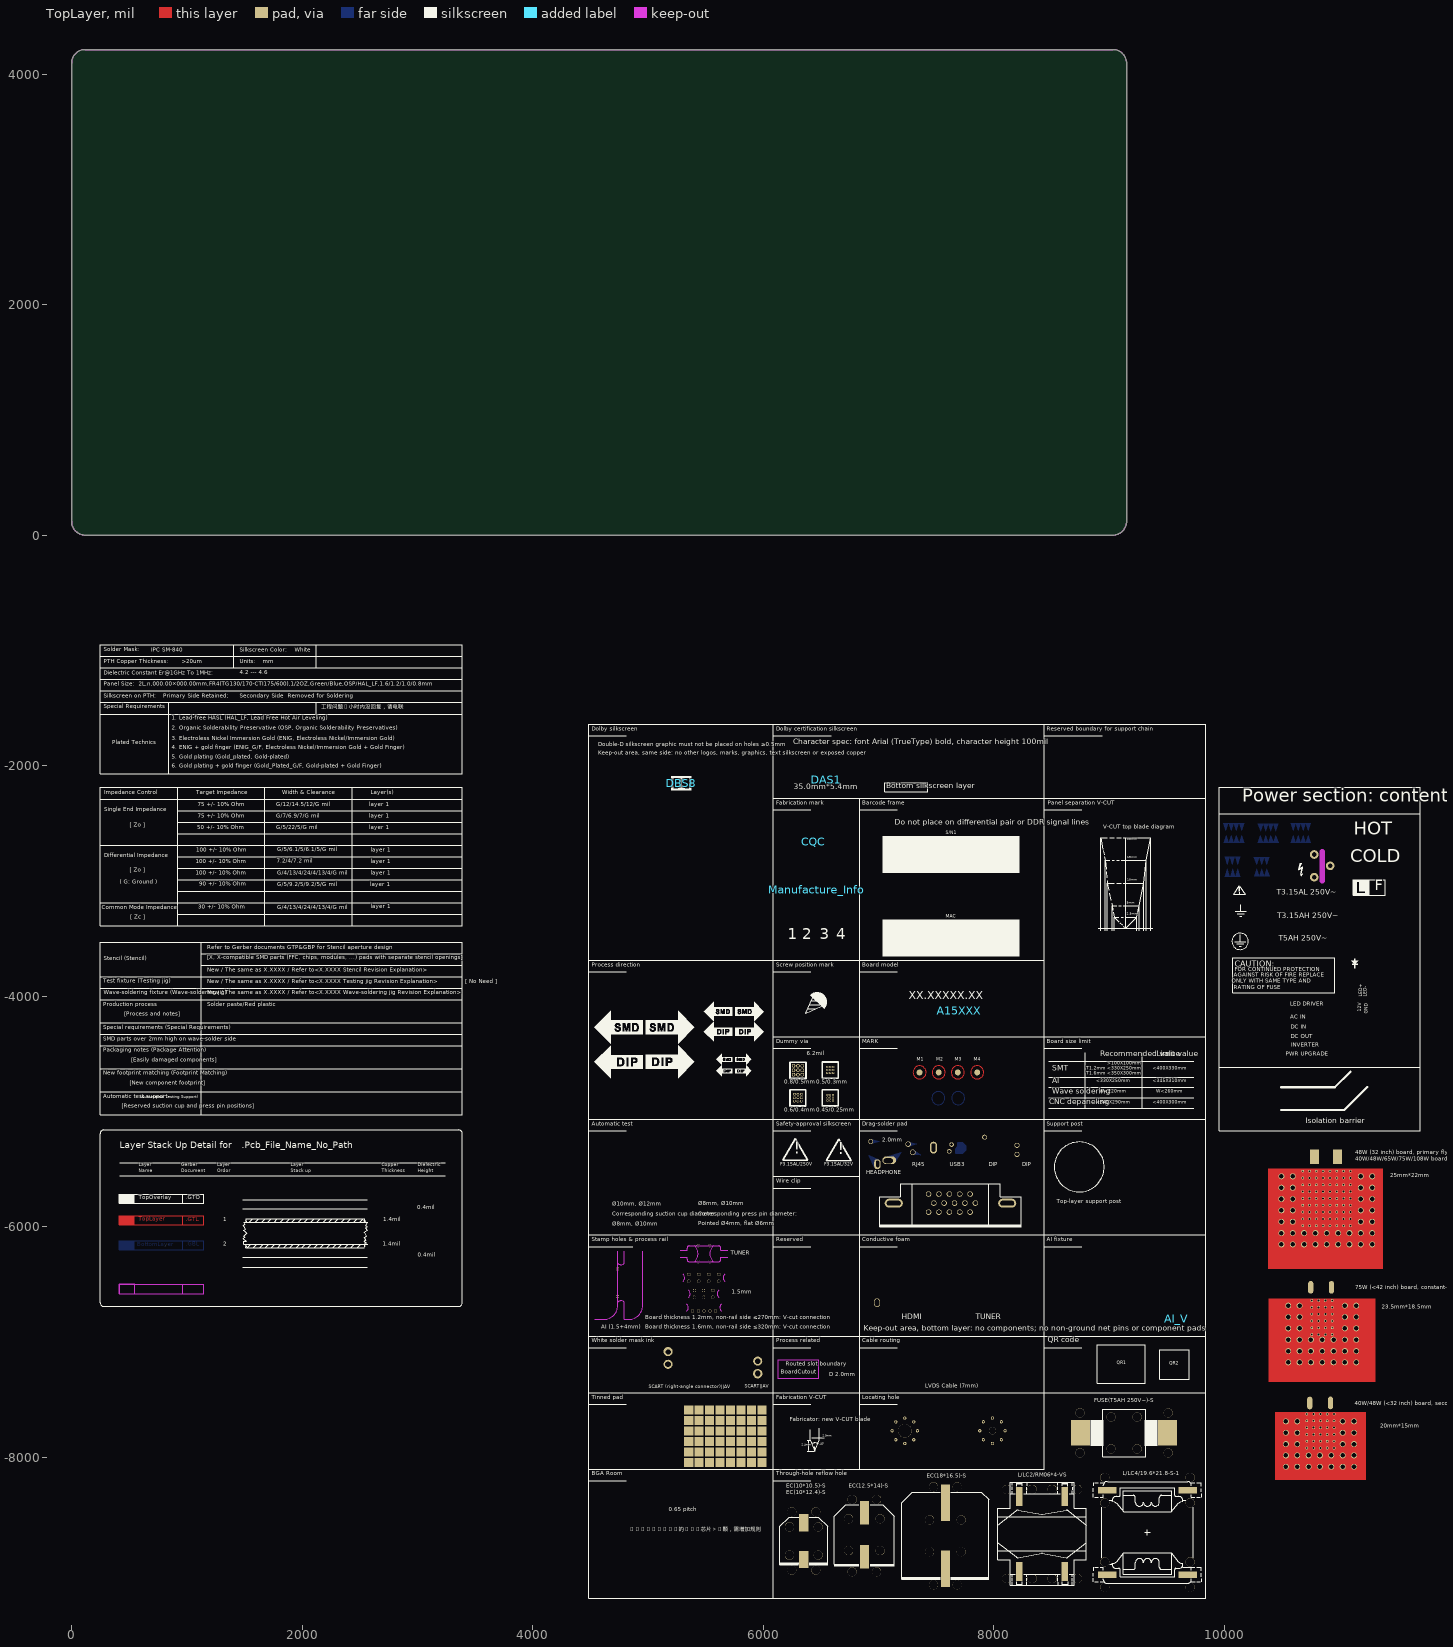
[diagram p0: TopLayer view]
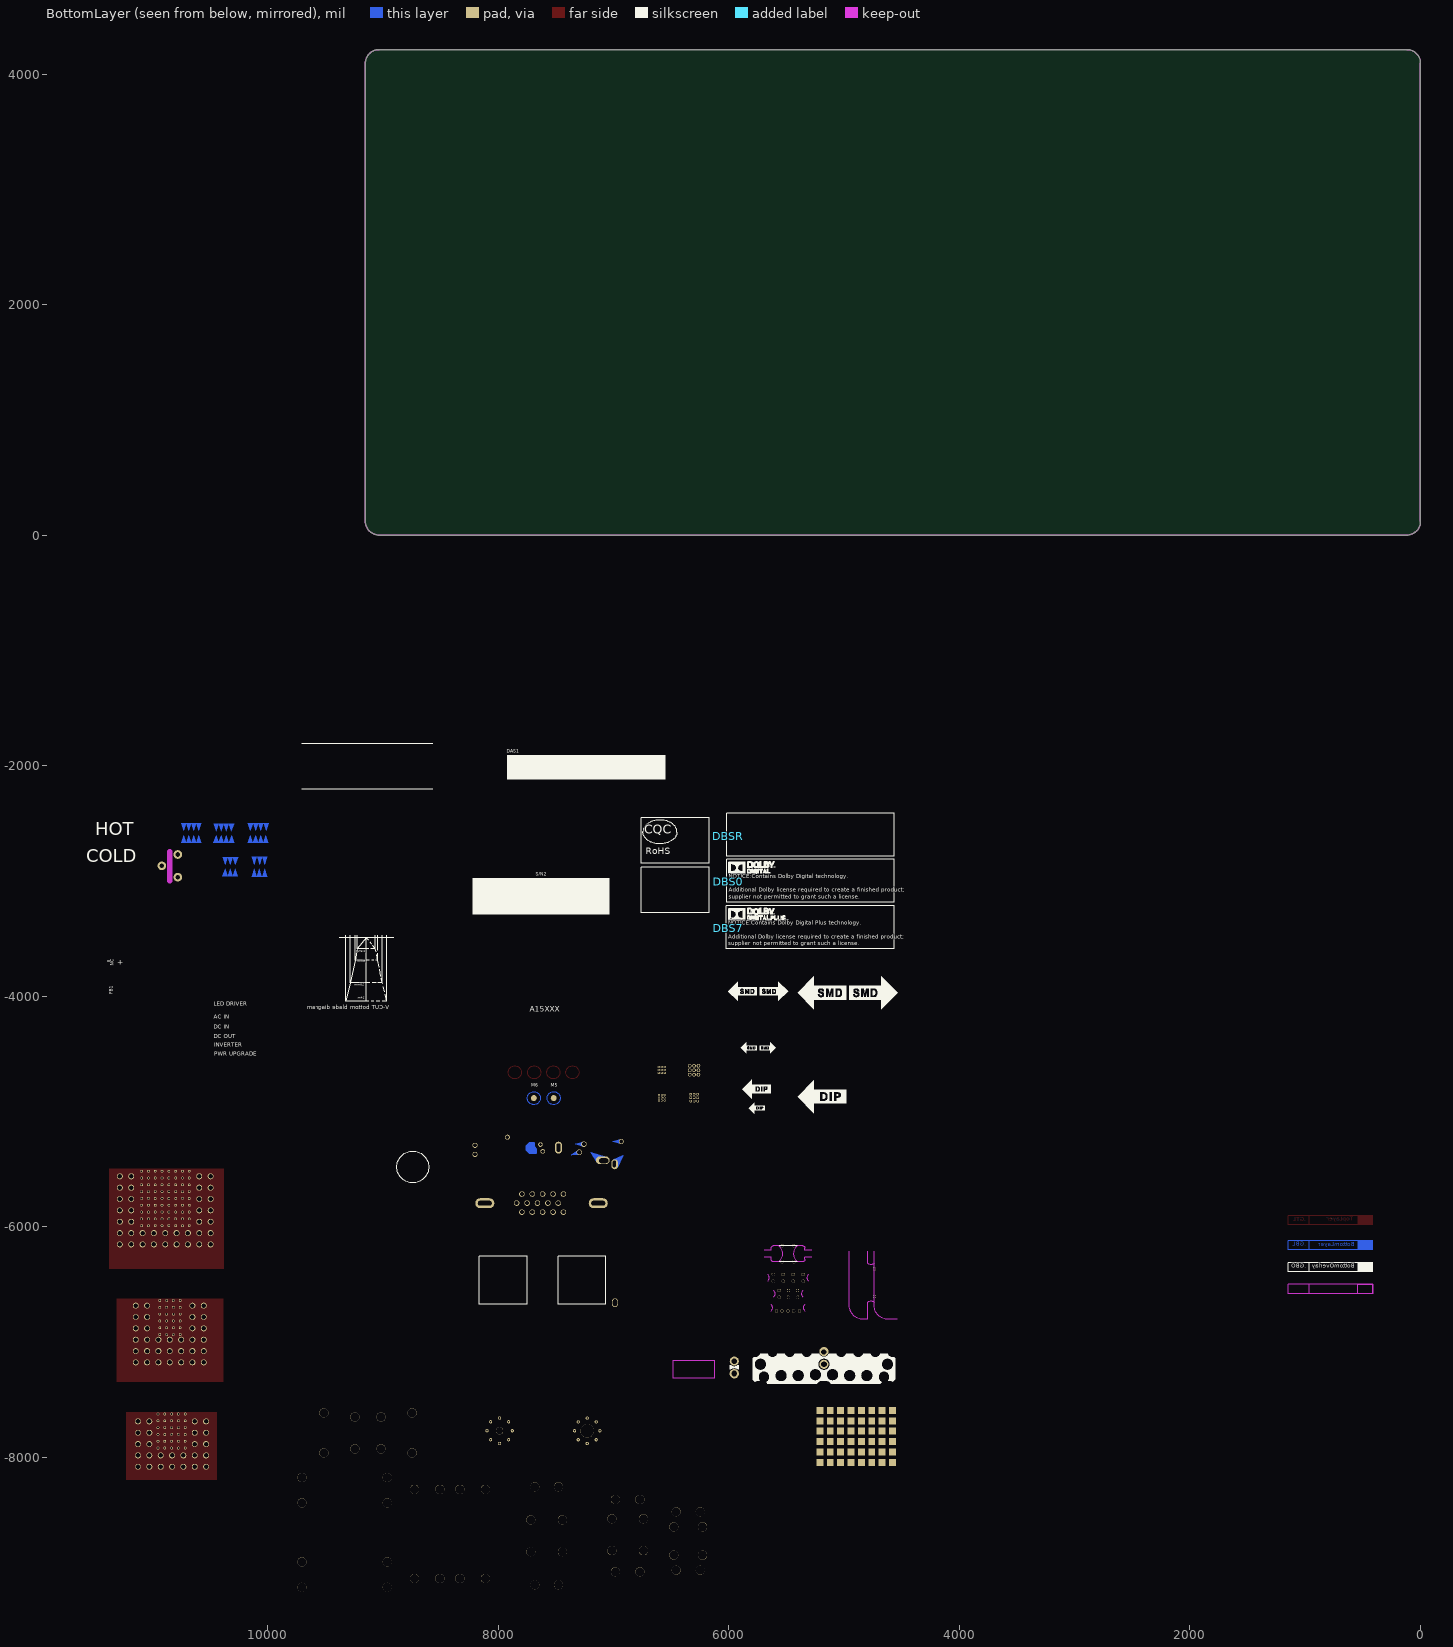
[diagram p1: BottomLayer view, seen from below]
# Altium PCB MISC86383.PcbDoc (part 1 of 2)
Units mil, origin at the board's own origin, x right, y up, seen from the top; angles counter-clockwise.
Board outline 9153.54 x 4212.6 mil, 2 copper layers (TopLayer, BottomLayer), stack 61.855 mil thick; 21 components, 2 nets, 540 pads, 0 vias.

## Layer stack, top to bottom
TopLayer: signal copper 1.4
Dielectric: core 59.055, FR-4, Dk 4.8
BottomLayer: signal copper 1.4

## Board outline
0,118.11 ccw(c118.11,118.11) 118.11,0 9035.43,0 9035.44,0 ccw(c9035.44,118.11) 9153.55,118.11 9153.55,4094.49 ccw(c9035.44,4094.49) 9035.44,4212.6 118.11,4212.6 ccw(c118.11,4094.49) 0,4094.49
cut-out: 6125.57,-7157.75 6125.57,-7314.38 6481.71,-7314.38 6481.71,-7157.75

## Design rules (kind name [scope] priority, off if disabled: settings)
Clearance ■KEEPOUT_18mil [(IsTrack Or IsArc) And (AsMM(Width) < 1) And IsKeepOut vs Not IsPad] p1: gap=18
Clearance ■HOT_7.2mm [InNetClass('HOT') vs InNetClass('All Nets') And (Not InNetClass('HOT'))] p2: gap=283.46
Clearance ■DFM_NPTH_10mil [(IsPadHoleValid And (PadIsPlated=false) Or IsPad And ((AsMM(PadXSize_AllLayers) < 1) or (AsMM(PadYSize_AllLayers) < 1 )) And IsKeepout) OR HasFootprintPad('ASSE*','0') vs Not IsPad] p3: gap=10
Clearance ■DFM_20mil [(IsTrack or IsArc or IsPad) And IsKeepOut vs IsTrack or IsArc or InPoly] p4: gap=20
Clearance ■C_RJ45_2mm [InNetClass('RJ45') vs Not InNetClass('RJ45') AND InNet('*')] p5: gap=78.74
Clearance ■VIA2VIA_6.2mil [(IsVia OR InPadClass('VIA5')) And Not ((IsVia OR InPadClass('VIA5')) And (AsMM(HoleDiameter) = 0.1)) vs (IsVia OR InPadClass('VIA5')) And Not ((IsVia OR InPadClass('VIA5')) And (AsMM(HoleDiameter) = 0.1))] p6: gap=6.2
Clearance ■V2V_BGA0p65_9p8mil [((IsVia OR InPadClass('VIA5')) And Not ((IsVia OR InPadClass('VIA5')) And (AsMM(HoleDiameter) = 0.1))) And (WithInRoom('BGA0p65-1') OR WithInRoom('BGA0p65-2')) vs ((IsVia OR InPadClass('VIA5')) And Not ((IsVia OR InPadClass('VIA5')) And (AsMM(HoleDiameter) = 0.1))) And (WithInRoom('BGA0p65-1') OR WithInRoom('BGA0p65-2'))] p7: gap=9.8
Clearance ■VIA2VIA_10.2mil [((IsVia OR InPadClass('VIA5')) And Not ((IsVia OR InPadClass('VIA5')) And (AsMM(HoleDiameter) = 0.1))) And Not (WithInRoom('BGA0p65-1') OR WithInRoom('BGA0p65-2')) vs ((IsVia OR InPadClass('VIA5')) And Not ((IsVia OR InPadClass('VIA5')) And (AsMM(HoleDiameter) = 0.1))) And Not (WithInRoom('BGA0p65-1') OR WithInRoom('BGA0p65-2'))] p8: gap=10.2
Clearance ■PWR_A12_8mil [((InNetClass('PWR_A12_8mil') or InNet('*12V*') or InNet('*24V*') or InNet('*PVCC*') or InNet('*19V*') or InNet('*AMP*POWER*') or InNet('*AMP*VCC*') or InNet('*LNB*')) And Not InNetClass('A12_8mil_EXC')) and Not IsPad vs Not InPoly] p9: gap=8
Clearance ■PS_L2All_3.2mm [InNet('L-1') vs InNet('*')] p10: gap=125.98
Clearance ■PS_L2LN_1.5mm [InNet('L') Or InNet('L-2') Or InNet('L-3') Or InNet('L-4') Or InNet('L-5') Or InNet('L-6') vs InNet('L-N') And Not(InNet('L') Or InNet('L-2') Or InNet('L-3') Or InNet('L-4') Or InNet('L-5') Or InNet('L-6'))] p11: gap=59.06
Clearance ■PS_N2LN_1.5mm [InNet('N') OR InNet('N-1') OR InNet('N-2') OR InNet('N-3') OR InNet('N-4') OR InNet('N-5') OR InNet('N-6') vs InNet('L-N') And Not (InNet('N') OR InNet('N-1') OR InNet('N-2') OR InNet('N-3') OR InNet('N-4') OR InNet('N-5') OR InNet('N-6'))] p12: gap=59.06
Clearance ■PS_L2LN_3mm [InNet('L') Or InNet('L-2') Or InNet('L-3') Or InNet('L-4') Or InNet('L-5') Or InNet('L-6') vs InNet('*') And Not (InNet('L-N') Or InNet('L') Or InNet('L-2') Or InNet('L-3') Or InNet('L-4') Or InNet('L-5') Or InNet('L-6') Or OnLayer('KeepOutLayer'))] p13: gap=118.11
Clearance ■PS_N2LN_3mm [InNet('N') OR InNet('N-1') OR InNet('N-2') OR InNet('N-3') OR InNet('N-4') OR InNet('N-5') OR InNet('N-6') vs InNet('*') And Not (InNet('L-N') Or InNet('N') OR InNet('N-1') OR InNet('N-2') OR InNet('N-3') OR InNet('N-4') OR InNet('N-5') OR InNet('N-6') Or OnLayer('KeepOutLayer'))] p14: gap=118.11
Clearance ■SIP2GND_8mil [HasFootprint('SIP*') vs InPoly] p15: gap=8
Clearance ■C_BGA_0P65 [HasFootprint('BGA*0.65*') vs InPoly] p16: gap=5
Clearance ■C_BGA_0P8 [HasFootprint('BGA*0.8*') vs InPoly] p17: gap=5.5
Clearance ■Poly_4mil [InPolygonClass('Poly_4mil') vs Not InPoly] p18: gap=4
Clearance ■Poly_5mil [InPolygonClass('Poly_5mil') vs Not InPoly] p19: gap=5
Clearance ■Poly_6.2mil [InPolygonClass('Poly_6.2mil') vs Not InPoly] p20: gap=6.2
Clearance ■Poly_8mil [InPolygonClass('Poly_8mil') vs Not InPoly] p21: gap=8
Clearance ■C_RFGND_1.8mm [InNet('RFGND') vs Not (InNet('RF*IN*') OR((IsTrack Or IsArc) And (AsMils(Width) < 6) And IsKeepOut) OR InNet('NetCT28*'))] p22: gap=70.87
Clearance ■ESD_10mil [HasFootprint('*IEC*') Or HasFootprint('*-F1*') Or HasFootprint('ANT-RF*')] p23: gap=10
Clearance ■ESD_20mil [HasFootprint('*SHIELD*')] p24: gap=20
Clearance ■GND_12mil [InNet('GND') vs InPoly] p25: gap=12
Clearance ■ESD_30mil [(HasFootprint('SCART*') OR HasFootprint('AV*') OR HasFootprint('DB15*') OR HasFootprint('PHONE*')) vs OnBottomLayer] p26: gap=30
Clearance ■ESD_NT_30mil [HasFootprint('SCART*') Or HasFootprint('PHONE-HD-12') Or HasFootprint('PHONE-HD-17') Or HasFootprint('PHONE-HD-10') Or HasFootprint('PHONE-HD-26') vs InNet('GND') And OnTopLayer] p27: gap=30
Clearance ■DFM_TH_5mil [HasFootprint('GND') or HasFootprint('TP*') or HasFootprint('MARK*') or HasFootprint('SPARK_GAP') or HasFootprint('USB-HD-3-2') or HasFootprint('PHONE-HS-20') and Not IsRegion vs OnBottomlayer And IsPad OR IsPadHoleValid] p28: gap=5
Clearance ■DFM_HS60_5mil [InPadClass('HS60') vs InPadClass('HS60') OR IsPadHoleValid and not InPadClass('VIA5')] p29: gap=5
Clearance ■DFM_BCR_4mm [IsPadHoleValid vs IsBoardCutoutRegion] p30: gap=157.48
Clearance ■DFM_TH_4mm [OnBottomlayer And IsSMTPin vs IsPadHoleValid and not InPadClass('VIA5')] p31: gap=157.48
Clearance ■DFM_HS60_4mm [InPadClass('HS60') vs IsPad and OnBottomlayer] p32: gap=157.48
Clearance ■V2P_BGA0p65_4p7mil [HasFootprint('BGA*') and IsPad And (WithInRoom('BGA0p65-1') OR WithInRoom('BGA0p65-2')) vs (IsVia OR InPadClass('VIA5')) And Not (IsVia And (AsMM(HoleDiameter) = 0.1))] p33: gap=4.7
Clearance ■VIA2PAD_BGA_5mil [(HasFootprint('BGA*') and IsPad) And Not (WithInRoom('BGA0p65-1') OR WithInRoom('BGA0p65-2')) vs (IsVia OR InPadClass('VIA5')) And Not (IsVia And (AsMM(HoleDiameter) = 0.1))] p34: gap=5
Clearance ■VIA2PAD_6mil [(IsVia OR InPadClass('VIA5')) And Not ((IsVia OR InPadClass('VIA5')) And (AsMM(HoleDiameter) = 0.1)) vs IsPad And Not HasFootprintPad('*','EPAD') and Not HasFootprintPad('*','257') and Not HasFootprintPad('TP','*') and Not HasFootprintPad('GND','JP*') and Not HasFootprintPad('LQFP216/0.4-2','217') and Not HasFootprintPad('QFP16*','17') and Not HasFootprintPad('QFN16*','17') and Not HasFootprintPad('QFN20*','21') and Not HasFootprintPad('QFN24*','25') and Not HasFootprintPad( 'QFN24*','29') and Not HasFootprintPad('QFN28*','29') and Not HasFootprintPad('QFN32*','33') and Not HasFootprintPad('QFN36*','37') and Not HasFootprintPad('QFN36*','0') and Not HasFootprintPad('QFN32*','0') and Not HasFootprintPad('QFN40*','41') and Not HasFootprintPad('QFN48*','49') and Not HasFootprintPad('LQFP48/0.5-2','49') and Not HasFootprintPad('*SSOP32*','33') and Not HasFootprintPad('SOP8*','9') and Not HasFootprintPad('WSON8/1.27*','9') and Not HasFootprintPad('DFN10/0.5-1*','11') and Not HasFootprintPad('SON16/0.4','9') and Not HasFootprintPad('MSOP10/0.5-1','11') and Not HasFootprintPad('QFN56/0.5','57') and Not HasFootprintPad('LGA31/0.5','3*') and Not InPadClass('VIA_HS60') and Not HasFootprintPad('TSSOP16/0.65-3','17') and Not HasFootprintPad('QFP128/0.5-2','129') and Not HasFootprintPad('QFP128/0.4-5','129') and Not HasFootprintPad('PQFP48*','49') and Not HasFootprintPad('QFP156/0.4-1','157') and Not HasFootprintPad('D2PAK3-TO-252','2') and Not HasFootprintPad('D2PAK3','2')] p35: gap=6
Clearance ■PAD2VIA5_6mil [(IsPad And Not (WithInRoom('BGA0p65-1') OR WithInRoom('BGA0p65-2'))) And ((AsMM(PadXSize_AllLayers) < 2.5) or ((AsMM(PadYSize_AllLayers) < 2.5))) And Not InPadclass('HS60') vs InPadClass('VIA5')] p36: gap=6
Clearance "■12mil for Polygon" [InPoly] p37: gap=12
Clearance 8mil [All] p38 off: gap=8
Clearance 7mil [All] p39 off: gap=7
Clearance 6.2mil [All] p40 off: gap=6.2
Clearance 6mil [All] p41: gap=6
Clearance 5.8mil [All] p42 off: gap=5.8
Clearance 5mil [Not ((IsTrack Or IsArc) And (Layer = 'KeepOutLayer')) vs Not (IsPad or ((IsTrack Or IsArc) And (Layer = 'KeepOutLayer')))] p43 off: gap=5
Clearance 4.5mil [Not ((IsTrack Or IsArc) And (Layer = 'KeepOutLayer')) vs Not (IsPad or ((IsTrack Or IsArc) And (Layer = 'KeepOutLayer')))] p44 off: gap=4.5
Clearance "4mil for Minimum" [Not ((IsTrack Or IsArc) And (Layer = 'KeepOutLayer')) vs Not (IsPad or ((IsTrack Or IsArc) And (Layer = 'KeepOutLayer')))] p45 off: gap=4
ComponentClearance ■DFMC_1mm [Not (InComponentClass('Co-Layout') Or HasFootprint('GND')) And (HasFootprint('T/E*') Or HasFootprint('T/PQ*') Or HasFootprint('USB*') Or HasFootprint('HDMI*') Or HasFootprint('USB*') Or HasFootprint('DC-*') Or HasFootprint('AV*') Or HasFootprint('ANT*') Or HasFootprint('PHONE*') Or HasFootprint('CICARD*') Or HasFootprint('CARD*') Or HasFootprint('DVI*') Or HasFootprint('DB*') Or HasFootprint('DP*') Or HasFootprint('DISPLAYPORT*') Or HasFootprint('OPTICAL*') Or HasFootprint('SCART*') Or HasFootprint('RJ45*') Or HasFootprint('USB*') Or HasFootprint('T-*') Or HasFootprint('T/*') Or HasFootprint('200-*') Or HasFootprint('ZhiJia*') Or HasFootprint('Dianpian*') Or HasFootprint('TanPian*') Or HasFootprint('P(*')) vs Not (InComponentClass('Co-Layout') Or HasFootprint('GND'))] p1 off: gap=39.37 collisioncheckmode=3 verticalgap=39.37 showdistances=FALSE
ComponentClearance ■DFMC_0.5mm [Not (InComponentClass('Co-Layout') Or HasFootprint('SO-23') Or HasFootprint('DIODE-s0402') Or HasFootprint('GND')) And (HasFootprint('M-*') Or HasFootprint('BGA*') Or HasFootprint('QFP*') Or HasFootprint('QFN*') Or HasFootprint('*DFN*') Or HasFootprint('*SOP*') Or HasFootprint('LGA*') Or HasFootprint('SOIC*') Or HasFootprint('EC*') Or HasFootprint('AC-*') Or HasFootprint('DIODE*') Or HasFootprint('XTAL*') Or HasFootprint('SO-*') Or HasFootprint('L/LC*') Or HasFootprint('L(*') Or HasFootprint('WIFI*') Or HasFootprint('SATA*') Or HasFootprint('POGO*') Or HasFootprint('SOT-223') Or HasFootprint('TO-252') Or HasFootprint('TO-263') Or HasFootprint('KEY*') Or HasFootprint('SW*') Or HasFootprint('DIP*') Or HasFootprint('SIP*') Or HasFootprint('DIP*') Or HasFootprint('CON*') Or HasFootprint('FFC*') Or HasFootprint('FPC*') Or HasFootprint('GDT*') Or HasFootprint('R2512*') Or HasFootprint('R2725*') Or HasFootprint('L2012*') Or HasFootprint('L2520*')) vs Not (InComponentClass('Co-Layout') Or HasFootprint('SO-23') Or HasFootprint('DIODE-s0402') Or HasFootprint('GND'))] p2 off: gap=19.68 collisioncheckmode=3 verticalgap=19.68 showdistances=FALSE
ComponentClearance ■DFMC_0.4mm [Not (InComponentClass('Co-Layout') Or HasFootprint('GND')) And (HasFootprint('C0201*') Or HasFootprint('C0402*') Or HasFootprint('C0603*') Or HasFootprint('C0805*') Or HasFootprint('C1206*') Or HasFootprint('C1210*') Or HasFootprint('R0201*') Or HasFootprint('R0402*') Or HasFootprint('R0603*') Or HasFootprint('R0805*') Or HasFootprint('R*0402*') Or HasFootprint('L0201*') Or HasFootprint('L0402*') Or HasFootprint('L0603*') Or HasFootprint('L0805*') Or HasFootprint('L1206*') Or HasFootprint('DIODE-s0402')) vs Not (InComponentClass('Co-Layout') Or HasFootprint('GND')) And (HasFootprint('C0201*') Or HasFootprint('C0402*') Or HasFootprint('C0603*') Or HasFootprint('C0805*') Or HasFootprint('C1206*') Or HasFootprint('C1210*') Or HasFootprint('R0201*') Or HasFootprint('R0402*') Or HasFootprint('R0603*') Or HasFootprint('R0805*') Or HasFootprint('R*0402*') Or HasFootprint('L0201*') Or HasFootprint('L0402*') Or HasFootprint('L0603*') Or HasFootprint('L0805*') Or HasFootprint('L1206*') Or HasFootprint('DIODE-s0402'))] p3 off: gap=15.75 collisioncheckmode=3 verticalgap=15.75 showdistances=FALSE
ComponentClearance ■DFMC_0.36mm [Not (InComponentClass('Co-Layout') Or HasFootprint('GND')) And HasFootprint('R1206*') vs Not (InComponentClass('Co-Layout') Or HasFootprint('GND')) And HasFootprint('R1206*')] p4 off: gap=14.17 collisioncheckmode=3 verticalgap=14.17 showdistances=FALSE
ComponentClearance ■DFMC_0.25mm [Not (InComponentClass('Co-Layout') Or HasFootprint('GND')) vs Not (InComponentClass('Co-Layout') Or HasFootprint('GND'))] p5 off: gap=9.84 collisioncheckmode=3 verticalgap=9.84 showdistances=FALSE
DiffPairsRouting ■DiffPair_USB_DiffPairsRouting [InDifferentialPairClass('USB')] p1: maxlimit=5 minlimit=4 mostfreqgap=5 maxuncoupledlength=200
DiffPairsRouting ■DiffPair_LVDS_DiffPairsRouting [InDifferentialPairClass('LVDS')] p2: maxlimit=5 minlimit=4 mostfreqgap=5 maxuncoupledlength=500
DiffPairsRouting ■DiffPair_HDMI_DiffPairsRouting [InDifferentialPairClass('HDMI')] p3: maxlimit=5 minlimit=4 mostfreqgap=5 maxuncoupledlength=200
DiffPairsRouting [All] p4: maxlimit=10 minlimit=10 mostfreqgap=10 maxuncoupledlength=500
FabricationTestPointUsage TestPointUsage [All] p1: valid=0 allowmultiple=FALSE
FabricationTestpoint Testpoint [All] p1: side=3 testpointundercomponent=TRUE minsize=40 maxsize=100 preferedsize=60 minholesize=20 maxholesize=40 preferedholesize=32 testpointgrid=1 allowsidetop=TRUE allowsidebottom=TRUE usegrid=TRUE gridtolerance=0.01
HoleSize HoleSize_VIA [ISVIA] p1 off: absolutevalues=TRUE maxlimit=23.62 minlimit=7.87 maxpercent=80.000 minpercent=20.000
HoleToHoleClearance Hole2Hole [All] p1 off: gap=18 allowstackedmicrovias=FALSE
MatchedLengths DiffPair_USB_MatchedLengths [InDifferentialPairClass('USB')] p1: tolerance=100 checknetsindiffpair=TRUE checkdiffpairvsdiffpair=TRUE checkothers=TRUE
MatchedLengths DiffPair_LVDS_MatchedLengths [InDifferentialPairClass('LVDS')] p2: tolerance=100 checknetsindiffpair=TRUE checkdiffpairvsdiffpair=TRUE checkothers=TRUE
MatchedLengths DiffPair_HDMI_MatchedLengths [InDifferentialPairClass('HDMI')] p3: tolerance=100 checknetsindiffpair=TRUE checkdiffpairvsdiffpair=TRUE checkothers=TRUE
MinimumAnnularRing [All] p1: minimumring=3.94
MinimumSolderMaskSliver ■MiniSolderMaskSliver [All] p1 off: minsoldermaskwidth=3.87
NetAntennae [Not (HasFootprint('ANT-7') or HasFootprint('ANT-BLUECORE'))] p1: netantennaetolerance=40
PermittedLayers [All] p1: toplayerpermitted=TRUE bottomlayerpermitted=TRUE
PlaneClearance ■Plane_ESD_30mil [(HasFootprint('SCART*') OR HasFootprint('AV*') OR HasFootprint('DB15*') OR HasFootprint('PHONE*'))] p1: clearance=30
PlaneClearance ■Plane_All_9mil [All] p2: clearance=9
PlaneConnect ■PlaneOverAll [IsVia or InPadClass('VIA5') Or HasFootprint('ASSE*') OR InPadclass('HS60')] p1: planeconnectstyle=Direct reliefexpansion=20 reliefentries=4 reliefconductorwidth=10 reliefairgap=10
PlaneConnect ■PlaneConnect [All] p2: planeconnectstyle=Relief reliefexpansion=12 reliefentries=4 reliefconductorwidth=30 reliefairgap=12
PolygonConnect ■PourOverAll [IsVia Or InPadclass('HS60') Or InPadClass('VIA5') Or HasFootprint('ASSE*') Or HasFootprint('DIODE-S0402') Or HasFootprint('RCL0524P') Or HasFootprint('SOT-89') OR HasFootprint('SOT-223') OR HasFootprint('TO-252') OR HasFootprint('TO-263') OR HasFootprint('DIODE') OR HasFootprint('SW-HS-2') OR HasFootprint('HDMI*') OR HasFootprint('SO-8B') OR HasFootprint('GND') OR HasFootprint('PHONE*') OR HasFootprint('DIP18/2.54-2') OR HasFootprint('DIP18/2.54-1') OR HasFootprint('UFL-R-SMT-1') OR HasFootprint('WIFI') OR HasFootprint('UM02BS') OR HasFootprint('*SCART*') OR HasFootprint('TSOT23-8/0.65') OR HasFootprint('*SOT-23-*') OR HasFootprint('SOP23-5-1') OR HasFootprint('SOP6/0.95') OR HasFootprint('M-WIFI-2-M603USA1') OR HasFootprint('M-MT7632U') OR HasFootprint('SOP8/1.27') OR HasFootprint('SOP8/1.27-3') OR HasFootprint('TSOT23-6') vs IsPolygon] p1: connectstyle=Direct reliefconductorwidth=10 reliefentries=4 polygonreliefangle="90 Angle"
PolygonConnect ■BGA_0P65 [HasFootprint('BGA*0.65*') vs IsPoly] p2: connectstyle=Relief reliefconductorwidth=8 reliefentries=4 polygonreliefangle="45 Angle"
PolygonConnect ■BGA_0P8 [HasFootprint('BGA*0.8*') vs IsPoly] p3: connectstyle=Relief reliefconductorwidth=9 reliefentries=4 polygonreliefangle="45 Angle"
PolygonConnect ■Polygon_RFGND [InNet('RFGND')] p4: connectstyle=Direct reliefconductorwidth=10 reliefentries=4 polygonreliefangle="90 Angle"
PolygonConnect ■ESD_SCART [HasFootprint('SCART*') vs IsPolygon And onBottomlayer] p5: connectstyle=Direct reliefconductorwidth=30 reliefentries=4 polygonreliefangle="90 Angle"
PolygonConnect ■C2Polygon_35mil [HasFootprint('EC*') vs IsPolygon] p6: connectstyle=Relief reliefconductorwidth=35 reliefentries=4 polygonreliefangle="90 Angle"
PolygonConnect ■C2Polygon_30mil [(HasFootprint('*0805*') OR HasFootprint('*1206*')) vs IsPolygon] p7: connectstyle=Relief reliefconductorwidth=30 reliefentries=4 polygonreliefangle="90 Angle"
PolygonConnect ■C2Polygon_25mil [HasFootprint('*0603*') Or IsThruPin vs IsPolygon] p8: connectstyle=Relief reliefconductorwidth=25 reliefentries=4 polygonreliefangle="90 Angle"
PolygonConnect ■C2Polygon_12mil [IsSMTPin vs IsPolygon] p9: connectstyle=Relief reliefconductorwidth=12 reliefentries=4 polygonreliefangle="90 Angle"
RoomDefinition BGA0p65-2 [All] p1: confinementstyle=ConfineOut formatcopy=TRUE lockcomponents=FALSE outline 5437.5,-8327.5 5867,-8327.5 5867,-8591 5437.5,-8591
RoomDefinition BGA0p65-1 [All] p2: confinementstyle=ConfineOut formatcopy=TRUE lockcomponents=FALSE outline 4715,-8327.5 5144.5,-8327.5 5144.5,-8591 4715,-8591
RoutingVias 0.6_0.4 [All] p1: holewidth=15.75 width=23.62 viastyle="Through Hole" minholewidth=15.75 minwidth=23.62 maxholewidth=15.75 maxwidth=23.62
RoutingVias 0.8_0.5 [All] p2 off: holewidth=19.68 width=31.5 viastyle="Through Hole" minholewidth=19.68 minwidth=31.5 maxholewidth=19.68 maxwidth=31.5
RoutingVias 0.5_0.3 [All] p3 off: holewidth=11.81 width=19.68 viastyle="Through Hole" minholewidth=11.81 minwidth=19.68 maxholewidth=11.81 maxwidth=19.68
RoutingVias 0.45_0.25 [All] p4 off: holewidth=9.84 width=17.72 viastyle="Through Hole" minholewidth=9.84 minwidth=17.72 maxholewidth=9.84 maxwidth=17.72
RoutingVias 0.4_0.2 [All] p5 off: holewidth=7.87 width=15.75 viastyle="Through Hole" minholewidth=7.87 minwidth=15.75 maxholewidth=7.87 maxwidth=15.75
RoutingVias 0.25_0.1 [All] p6 off: holewidth=3.94 width=9.84 viastyle="Through Hole" minholewidth=3.94 minwidth=9.84 maxholewidth=3.94 maxwidth=9.84
SMDNeckDown ■SMDNeckDown_Chip [HasFootprint('FFC*') or HasFootprint('QFP*') or HasFootprint('QFN*') or HasFootprint('HDMI*') or HasFootprint('BGA*')] p1: percent=100.000
SMDToCorner [All] p1 off: distance=40000
ShortCircuit ■ShortCircuit_JP [HasFootprintPad( 'GND','JP_1K') vs HasFootprintPad( 'GND','JP_2K')] p1: allowed=TRUE
ShortCircuit ■ShortCircuit_ViaOnEpad [HasFootprintPad( '*','EPAD') vs IsVia AND InNet('*')] p2: allowed=TRUE
ShortCircuit ■ShortCircuit_R0402 [HasFootprintPad('R0402SC','1') OR HasFootprintPad('R0402SC','2') vs HasFootprintPad('R0402SC','3')] p3: allowed=TRUE
ShortCircuit ■ShortCircuit_RP2_0402 [HasFootprintPad('RP2*0402-1SC','1') OR HasFootprintPad('RP2*0402-1SC','2') vs HasFootprintPad('RP2*0402-1SC','5')] p4: allowed=TRUE
ShortCircuit ■ShortCircuit_RP2-0402 [HasFootprintPad('RP2*0402-1SC','3') OR HasFootprintPad('RP2*0402-1SC','4') vs HasFootprintPad('RP2*0402-1SC','6')] p5: allowed=TRUE
ShortCircuit ■ShortCircuit_LC4_SC1 [HasFootprintPad('L/LC4/0.85*0.65SC','1') OR HasFootprintPad('L/LC4/0.85*0.65SC','2') vs HasFootprintPad('L/LC4/0.85*0.65SC','5')] p6: allowed=TRUE
ShortCircuit ■ShortCircuit_LC4-SC1 [HasFootprintPad('L/LC4/0.85*0.65SC','3') OR HasFootprintPad('L/LC4/0.85*0.65SC','4') vs HasFootprintPad('L/LC4/0.85*0.65SC','5')] p7: allowed=TRUE
ShortCircuit ■ShortCircuit_R0603 [HasFootprintPad('R0603SC','1') OR HasFootprintPad('R0603SC','2') vs HasFootprintPad('R0603SC','3')] p8: allowed=TRUE
ShortCircuit ■ShortCircuit_R0805 [HasFootprintPad('R0805SC','1') OR HasFootprintPad('R0805SC','2') vs HasFootprintPad('R0805SC','3')] p9: allowed=TRUE
ShortCircuit ■ShortCircuit_L0805 [HasFootprintPad('L0805SC','1') OR HasFootprintPad('L0805SC','2') vs HasFootprintPad('L0805SC','3')] p10: allowed=TRUE
ShortCircuit ■ShortCircuit_R1206 [HasFootprintPad('R1206SC','1') OR HasFootprintPad('R1206SC','2') vs HasFootprintPad('R1206SC','3')] p11: allowed=TRUE
ShortCircuit ■ShortCircuit [InNet('*')] p12: allowed=FALSE
SilkToSilkClearance ■Silk2Silk [All] p1: silktosilkclearance=5
SilkscreenOverComponentPads ■SilkOverPads [IsText] p1: minsilkscreentomaskgap=0.1
SolderMaskExpansion ■SolderMask_VIA [IsVia] p1: expansion=5.1
SolderMaskExpansion ■SolderMask_All [All] p2: expansion=2
UnRoutedNet ■UnRoutedNet [All] p1:
ViasUnderSMD [All] p1: allowed=FALSE
Width ■Width_2.5mm [InFromToClass('Width_2.5mm')] p1: maxlimit=98.43 minlimit=98.43 preferedwidth=98.43
Width ■Width_1.5mm [InFromToClass('Width_1.5mm')] p2: maxlimit=59.06 minlimit=59.06 preferedwidth=59.06
Width ■DiffPair_USB_Width [InDifferentialPairClass('USB')] p3: maxlimit=11 minlimit=4 preferedwidth=11
Width ■DiffPair_LVDS_Width [InDifferentialPairClass('LVDS')] p4: maxlimit=7 minlimit=4 preferedwidth=7
Width ■DiffPair_HDMI_Width [InDifferentialPairClass('HDMI')] p5: maxlimit=7 minlimit=4 preferedwidth=7
Width [All] p6: maxlimit=500 minlimit=3 preferedwidth=8
14 further rules are at their usual default settings.

## Classes and differential pairs
pad class VIA5: Free-0 Free-VIA5 Free-via5
pad class HS60: Free-HS60

## Components (designator, comment, footprint, x,y, rotation, side; value= is the part's Value field where it differs from the comment)
A15XXX "PCB_TIME" PCB_TIME 7701.97,-4126.84 r90 top (schematic designator A13XX)
AI_V "Comment" AI_GRIPPER_V 9588,-6800 r270 top
CQC "CQC" CQC 6440.87,-2659.33 r0 top
DAS1 "35.0*5.4mm" DOLBY_AS2 6548.37,-2122.33 r0 top
DBS0 "DOLBY" DOLBY-SILK 6004.65,-3008.84 r180 bottom (schematic designator DOLBY)
DBS7 "DOLBY PLUS" "DOLBY PLUS-SILK" 6006.65,-3412.84 r180 bottom (schematic designator "DOLBY PLUS")
DBS8 "Comment" Double-D-SILK 5290,-2153.5 r0 top
DBSR "NO DOLBY" "NO DOLBY-SILK" 6004.31,-2611.18 r180 bottom
M1 "MARK" MARK 7357.31,-4661.68 r0 top
M2 "MARK" MARK 7523.31,-4661.68 r0 top
M3 "MARK" MARK 7689.31,-4661.68 r0 top
M4 "MARK" MARK 7857.31,-4661.68 r0 top
M5 "MARK" MARK 7520.31,-4884.68 r180 bottom
M6 "MARK" MARK 7692.31,-4884.68 r180 bottom
MAC "Comment" Barcode 7630,-3496 r0 top
Manufacture_Info "Manufacture_Info" Manufacture_Info 6466.87,-3077.33 r180 top
QR1 "Comment" QRCODE-1 9106.91,-7192.24 r0 top
QR2 "Comment" QRCODE-2 9568.91,-7194.24 r0 top
S/N1 "Comment" Barcode 7630,-2772 r0 top
S/N2 "Comment" Barcode 7630,-3134 r180 bottom
XX.XXXXX.XX "PCB_NAME" PCB_NAME 7420.97,-4045.84 r90 top

## Footprints (in the part's own frame and the unit in brackets; to place one, negate y for a bottom-side part, rotate by r counter-clockwise, add the part's x,y. Pads: shape width x height; smd on the part's side, far side on the other; paste and mask are expansions set on the pad)
AI_GRIPPER_V [mm] "3D shape for vertical type AI equipment"
  round 1.5 on Mech5: 0(0,-2.5) 1(0,0) 2(0,2.5)
  body extent -29.13,-4.7 2.5,4.7, height 54.74
Barcode [mm]
  round 0.3 on Mech2: 0(0,0)
  silkscreen extent -15,-4 15,4
CQC [mil]
"DOLBY PLUS-SILK" [mil]
  silkscreen extent -16,-177 1441,197
DOLBY-SILK [mil]
  silkscreen extent -16,-177 1441,197
DOLBY_AS2 [mil] "杜比认证预留框，两行印刷，规格35.0*5.4mm"
Double-D-SILK [mil] "Dolby Double-D Silkscreen"
  silkscreen extent -86,-60 86,60
Manufacture_Info [mm]
  round 0.3 on Mech2: 0(0,0)
MARK [mm] "SMD 使用"
  round 1.3 smd paste+0 mask+0.65: 0(0,0)
  TopLayer circle w0.254: c0,0 r1.444
  TopLayer pour cut-out: -1.3,0 -1.201,-0.497 -0.919,-0.919 -0.497,-1.201 0,-1.3 0,-1.3 0.497,-1.201 0.919,-0.919 1.201,-0.497 1.3,0 1.3,0 1.201,0.497 0.919,0.919 0.497,1.201 0,1.3 0,1.3 -0.497,1.201 -0.919,0.919 -1.201,0.497 -1.3,0
"NO DOLBY-SILK" [mil]
  silkscreen extent -16,-177 1441,197
PCB_NAME [mm]
  round 0.3 on Mech2: 0(0,0)
PCB_TIME [mm]
  round 0.3 on Mech2: 0(0,0)
QRCODE-1 [mm] "明码+暗码，标签大小10*8mm，视睿"
  round 0.3 on Mech2: 0(0,0)
  silkscreen extent -5.25,-4.25 5.25,4.25
QRCODE-2 [mm] "暗码，标签大小6*6mm，视睿"
  round 0.3 on Mech2: 0(0,0)
  silkscreen extent -3.25,-3.25 3.25,3.25

## Part data
DBS7: library part DOLBY
M1 M2 M3 M4 M5 M6: library part MARK-D

## Free pads (board coordinates)
  round 27.56 hole 27.56 unplated: 0(4737.96,-6605.22) 0(4737.96,-6366.72) 0(5588.2,-6732.15) VIA5(5356.16,-6473.4) VIA5(5356.16,-6414.35) VIA5(5388.2,-6732.15) VIA5(5403.66,-6611.9) VIA5(5403.66,-6552.85) VIA5(5436.95,-6304.36) VIA5(5436.95,-6166.56) VIA5(5438.2,-6732.15) VIA5(5442.77,-6473.4) VIA5(5442.77,-6414.35) VIA5(5483.97,-6611.9) VIA5(5483.97,-6552.85) VIA5(5488.2,-6732.15) VIA5(5529.39,-6473.4) VIA5(5529.39,-6414.35) VIA5(5536.95,-6304.36) VIA5(5536.95,-6166.56) VIA5(5538.2,-6732.15) VIA5(5564.29,-6611.9) VIA5(5564.29,-6552.85) VIA5(5616,-6473.4) VIA5(5616,-6414.35)
  round 157.48 on Keep-Out: 0(4757.65,-6486.76)
  round 137.8 on Keep-Out: 0(6463.47,-5871.84) 0(8743,-5482)
  round 78.74 on Keep-Out: 0(6664.87,-7207.33)
  round 43.31 hole 31.5: 0(6933.97,-5260.84) 29(8202.99,-5373.27) 30(7921.97,-5223.84) 30(8202.99,-5294.53)
  oval 51.18x74.8 hole 35.43 slot 59.06 at 90 deg: 0(6988.47,-6659.34)
  oval 165.35x86.61 on Top Overlay: 0(7133.61,-5796.63) 0(8117.86,-5796.63)
  round 47.24 hole 35.43: 0(7258.39,-5284.42) 0(7298.55,-5354.5) 1(7796.21,-5717.1) 2(7706.05,-5717.1) 3(7615.9,-5717.1) 4(7525.74,-5717.1) 5(7435.58,-5717.1) 6(7841.29,-5795.84) 7(7751.13,-5795.84) 8(7660.97,-5795.84) 9(7570.82,-5795.84) 10(7480.66,-5795.84) 11(7796.21,-5874.58) 12(7706.05,-5874.58) 13(7615.9,-5874.58) 14(7525.74,-5874.58) 15(7435.58,-5874.58)
  oval 62.99x102.36 hole 31.5 slot 70.87 at 90 deg: 0(7478.07,-5314.34)
  rect 86.61x163.39 on Top Paste: 0(8223.76,-8991.48) 0(8223.76,-8339.91) 0(8617.46,-8991.48) 0(8617.46,-8339.91)
  round 94.49 on Keep-Out: 0(8420.61,-8931.44) 0(8420.61,-8399.94) 0(9167.02,-8652.56) 0(9501.67,-8652.56)
  rect 196.85x196.85 on Top Overlay: 0(8665.41,-7197.74)
  rect 78.74x151.57 smd: 1(6352.98,-8566.93) 2(6352.98,-8887.8)
  rect 78.74x204.72 smd: 1(6878.62,-8482.31) 2(6878.62,-8864.2)
  rect 78.74x314.96 smd: 1(7581.78,-8395.85) 2(7581.78,-8968.68)
  rect 55.12x163.39 smd paste-98.43: 1(8223.76,-8991.48) 2(8617.46,-8991.48) 3(8617.46,-8339.91) 4(8223.76,-8339.91)
  rect 165.35x220.47 smd: 1(8753.64,-7789.75) 2(9509.78,-7789.75)
  rect 161.42x86.61 on Top Paste: 1(8985.92,-9018.7) 1(8985.92,-8286.42) 1(9682.77,-9018.7) 1(9682.77,-8286.42)
  rect 161.42x55.12 smd: 1(8985.92,-8286.4) 2(8985.92,-9018.68) 3(9682.77,-9018.68) 4(9682.77,-8286.4)
  rect 78.74x125.98 smd: 1(10983.29,-5394.97) 3(10783.29,-5394.97)
  round 78.74 hole 51.18: 3(5175.37,-7193.83)
  round 82.68 hole 51.18: 3(5953.37,-7275.63)
  oval 118.11x66.93 hole 39.37 slot 78.74 at 0 deg copper offset 8,4: 3(7086.41,-5428.24)
  oval 45x110 smd: 3(10743.23,-7530.31) 3(10751.19,-6527.01) 3(10922.82,-7529.35) 3(10930.79,-6526.05)
  round 39.37 hole 27.56: 4(7615.29,-5346.9) 5(7634.97,-5287.84)
  oval 55.12x86.61 hole 27.56 slot 55.12 at 90 deg copper offset -3,-3: 5(6994.09,-5455.8)
  round 78.74 hole 47.24 copper offset 0,3.94: 11(5175.37,-7087.53)
  round 78.74 hole 47.24: 11(5953.37,-7166.33)
  oval 157.48x78.74 / inner oval 157.48x78.74 / far side oval 165.35x86.61 hole 39.37 slot 118.11 at 0 deg: 16(7133.61,-5796.63) 17(8117.86,-5796.63)
  round 74.8 hole 39.37 unplated: D(10919.43,-2869.7) G(10781.63,-2771.28) S(10781.63,-2968.13)
  rect 60x60 smd far side paste-30 mask+0: HS60(4580.7,-8044.54) HS60(4580.7,-7954.54) HS60(4580.7,-7864.54) HS60(4580.7,-7774.54) HS60(4580.7,-7684.54) HS60(4580.7,-7594.54) HS60(4670.7,-8044.54) HS60(4670.7,-7954.54) HS60(4670.7,-7864.54) HS60(4670.7,-7774.54) HS60(4670.7,-7684.54) HS60(4670.7,-7594.54) HS60(4760.7,-8044.54) HS60(4760.7,-7954.54) HS60(4760.7,-7864.54) HS60(4760.7,-7774.54) HS60(4760.7,-7684.54) HS60(4760.7,-7594.54) HS60(4850.7,-8044.54) HS60(4850.7,-7954.54) HS60(4850.7,-7864.54) HS60(4850.7,-7774.54) HS60(4850.7,-7684.54) HS60(4850.7,-7594.54) HS60(4940.7,-8044.54) HS60(4940.7,-7954.54) HS60(4940.7,-7864.54) HS60(4940.7,-7774.54) HS60(4940.7,-7684.54) HS60(4940.7,-7594.54) HS60(5030.7,-8044.54) HS60(5030.7,-7954.54) HS60(5030.7,-7864.54) HS60(5030.7,-7774.54) HS60(5030.7,-7684.54) HS60(5030.7,-7594.54) HS60(5120.7,-8044.54) HS60(5120.7,-7954.54) HS60(5120.7,-7864.54) HS60(5120.7,-7774.54) HS60(5120.7,-7684.54) HS60(5120.7,-7594.54) HS60(5210.7,-8044.54) HS60(5210.7,-7954.54) HS60(5210.7,-7864.54) HS60(5210.7,-7774.54) HS60(5210.7,-7684.54) HS60(5210.7,-7594.54)
  rect 78.74x78.74 smd mask+0: HS60(5354.88,-8044.54) HS60(5354.88,-7953.98) HS60(5354.88,-7863.43) HS60(5354.88,-7772.88) HS60(5354.88,-7682.33) HS60(5354.88,-7591.78) HS60(5445.43,-8044.54) HS60(5445.43,-7953.98) HS60(5445.43,-7863.43) HS60(5445.43,-7772.88) HS60(5445.43,-7682.33) HS60(5445.43,-7591.78) HS60(5535.98,-8044.54) HS60(5535.98,-7953.98) HS60(5535.98,-7863.43) HS60(5535.98,-7772.88) HS60(5535.98,-7682.33) HS60(5535.98,-7591.78) HS60(5626.53,-8044.54) HS60(5626.53,-7953.98) HS60(5626.53,-7863.43) HS60(5626.53,-7772.88) HS60(5626.53,-7682.33) HS60(5626.53,-7591.78) HS60(5717.08,-8044.54) HS60(5717.08,-7953.98) HS60(5717.08,-7863.43) HS60(5717.08,-7772.88) HS60(5717.08,-7682.33) HS60(5717.08,-7591.78) HS60(5807.63,-8044.54) HS60(5807.63,-7953.98) HS60(5807.63,-7863.43) HS60(5807.63,-7772.88) HS60(5807.63,-7682.33) HS60(5807.63,-7591.78) HS60(5898.18,-8044.54) HS60(5898.18,-7953.98) HS60(5898.18,-7863.43) HS60(5898.18,-7772.88) HS60(5898.18,-7682.33) HS60(5898.18,-7591.78) HS60(5988.74,-8044.54) HS60(5988.74,-7953.98) HS60(5988.74,-7863.43) HS60(5988.74,-7772.88) HS60(5988.74,-7682.33) HS60(5988.74,-7591.78)
  round 78.74 hole 78.74 unplated: VIA5(6228.1,-8849.89) VIA5(6228.1,-8604.85) VIA5(6248.66,-8980.73) VIA5(6248.66,-8474) VIA5(6457.3,-8980.73) VIA5(6457.3,-8474) VIA5(6477.86,-8849.89) VIA5(6477.86,-8604.85) VIA5(6741.93,-8811.52) VIA5(6741.93,-8534.99) VIA5(6771.86,-8994.86) VIA5(6771.86,-8367.4) VIA5(6985.38,-8994.86) VIA5(6985.38,-8367.4) VIA5(7015.31,-8811.52) VIA5(7015.31,-8534.99) VIA5(7445.09,-8820.53) VIA5(7445.09,-8544) VIA5(7479.18,-9107.11) VIA5(7479.18,-8257.42) VIA5(7684.38,-9107.11) VIA5(7684.38,-8257.42) VIA5(7718.47,-8820.53) VIA5(7718.47,-8544) VIA5(8113.63,-9052.27) VIA5(8113.63,-8279.11) VIA5(8333.9,-9052.27) VIA5(8333.9,-8279.11) VIA5(8507.33,-9052.27) VIA5(8507.33,-8279.11) VIA5(8727.6,-9052.27) VIA5(8727.6,-8279.11) VIA5(8749.18,-7963.27) VIA5(8749.18,-7616.23) VIA5(8964.5,-9128.84) VIA5(8964.5,-8908.56) VIA5(8964.5,-8396.55) VIA5(8964.5,-8176.28) VIA5(9018.64,-7928.02) VIA5(9018.64,-7651.48) VIA5(9244.78,-7928.02) VIA5(9244.78,-7651.48) VIA5(9514.24,-7963.27) VIA5(9514.24,-7616.23) VIA5(9704.2,-9128.84) VIA5(9704.2,-8908.56) VIA5(9704.2,-8396.55) VIA5(9704.2,-8176.28)
  round 31.5 hole 19.68 paste-15.75 mask-15.75: VIA5(6264.36,-4681.07) VIA5(6264.36,-4643.07) VIA5(6264.36,-4605.07) VIA5(6302.36,-4681.07) VIA5(6302.36,-4643.07) VIA5(6302.36,-4605.07) VIA5(6340.36,-4681.07) VIA5(6340.36,-4643.07) VIA5(6340.36,-4605.07)
  round 23.62 hole 15.75 paste-15.75 mask-15.75: VIA5(6271.87,-4910.83) VIA5(6271.87,-4880.83) VIA5(6271.87,-4850.83) VIA5(6301.87,-4910.83) VIA5(6301.87,-4880.83) VIA5(6301.87,-4850.83) VIA5(6331.87,-4910.83) VIA5(6331.87,-4880.83) VIA5(6331.87,-4850.83) VIA5(10681.79,-5991.46) VIA5(10681.79,-5932.41) VIA5(10681.79,-5873.35) VIA5(10681.79,-5814.29) VIA5(10681.79,-5755.24) VIA5(10681.79,-5696.18) VIA5(10681.79,-5637.13) VIA5(10681.79,-5578.07) VIA5(10681.79,-5519.02) VIA5(10717.33,-7920.9) VIA5(10717.33,-7861.85) VIA5(10717.33,-7802.79) VIA5(10717.33,-7743.74) VIA5(10717.33,-7684.68) VIA5(10717.33,-7625.63) VIA5(10740.84,-5991.46) VIA5(10740.84,-5932.41) VIA5(10740.84,-5873.35) VIA5(10740.84,-5814.29) VIA5(10740.84,-5755.24) VIA5(10740.84,-5696.18) VIA5(10740.84,-5637.13) VIA5(10740.84,-5578.07) VIA5(10740.84,-5519.02) VIA5(10760.53,-6936.34) VIA5(10760.53,-6877.29) VIA5(10760.53,-6818.23) VIA5(10760.53,-6759.18) VIA5(10760.53,-6700.12) VIA5(10760.53,-6641.07) VIA5(10776.38,-7920.9) VIA5(10776.38,-7861.85) VIA5(10776.38,-7802.79) VIA5(10776.38,-7743.74) VIA5(10776.38,-7684.68) VIA5(10776.38,-7625.63) VIA5(10799.9,-5991.46) VIA5(10799.9,-5932.41) VIA5(10799.9,-5873.35) VIA5(10799.9,-5814.29) VIA5(10799.9,-5755.24) VIA5(10799.9,-5696.18) VIA5(10799.9,-5637.13) VIA5(10799.9,-5578.07) VIA5(10799.9,-5519.02) VIA5(10819.58,-6936.34) VIA5(10819.58,-6877.29) VIA5(10819.58,-6818.23) VIA5(10819.58,-6759.18) VIA5(10819.58,-6700.12) VIA5(10819.58,-6641.07) VIA5(10835.44,-7920.9) VIA5(10835.44,-7861.85) VIA5(10835.44,-7802.79) VIA5(10835.44,-7743.74) VIA5(10835.44,-7684.68) VIA5(10835.44,-7625.63) VIA5(10858.95,-5991.46) VIA5(10858.95,-5932.41) VIA5(10858.95,-5873.35) VIA5(10858.95,-5814.29) VIA5(10858.95,-5755.24) VIA5(10858.95,-5696.18) VIA5(10858.95,-5637.13) VIA5(10858.95,-5578.07) VIA5(10858.95,-5519.02) VIA5(10878.64,-6936.34) VIA5(10878.64,-6877.29) VIA5(10878.64,-6818.23) VIA5(10878.64,-6759.18) VIA5(10878.64,-6700.12) VIA5(10878.64,-6641.07) VIA5(10894.49,-7920.9) VIA5(10894.49,-7861.85) VIA5(10894.49,-7802.79) VIA5(10894.49,-7743.74) VIA5(10894.49,-7684.68) VIA5(10894.49,-7625.63) VIA5(10918.01,-5991.46) VIA5(10918.01,-5932.41) VIA5(10918.01,-5873.35) VIA5(10918.01,-5814.29) VIA5(10918.01,-5755.24) VIA5(10918.01,-5696.18) VIA5(10918.01,-5637.13) VIA5(10918.01,-5578.07) VIA5(10918.01,-5519.02) VIA5(10937.69,-6936.34) VIA5(10937.69,-6877.29) VIA5(10937.69,-6818.23) VIA5(10937.69,-6759.18) VIA5(10937.69,-6700.12) VIA5(10937.69,-6641.07) VIA5(10953.55,-7920.9) VIA5(10953.55,-7861.85) VIA5(10953.55,-7802.79) VIA5(10953.55,-7743.74) VIA5(10953.55,-7684.68) VIA5(10953.55,-7625.63) VIA5(10977.06,-5991.46) VIA5(10977.06,-5932.41) VIA5(10977.06,-5873.35) VIA5(10977.06,-5814.29) VIA5(10977.06,-5755.24) VIA5(10977.06,-5696.18) VIA5(10977.06,-5637.13) VIA5(10977.06,-5578.07) VIA5(10977.06,-5519.02) VIA5(11036.12,-5991.46) VIA5(11036.12,-5932.41) VIA5(11036.12,-5873.35) VIA5(11036.12,-5814.29) VIA5(11036.12,-5755.24) VIA5(11036.12,-5696.18) VIA5(11036.12,-5637.13) VIA5(11036.12,-5578.07) VIA5(11036.12,-5519.02) VIA5(11095.17,-5991.46) VIA5(11095.17,-5932.41) VIA5(11095.17,-5873.35) VIA5(11095.17,-5814.29) VIA5(11095.17,-5755.24) VIA5(11095.17,-5696.18) VIA5(11095.17,-5637.13) VIA5(11095.17,-5578.07) VIA5(11095.17,-5519.02)
  round 19.68 hole 11.81 paste-15.75 mask-15.75: VIA5(6556.37,-4666.33) VIA5(6556.37,-4640.33) VIA5(6556.37,-4614.33) VIA5(6582.37,-4666.33) VIA5(6582.37,-4640.33) VIA5(6582.37,-4614.33) VIA5(6608.37,-4666.33) VIA5(6608.37,-4640.33) VIA5(6608.37,-4614.33)
  round 17.72 hole 9.84 paste-15.75 mask-15.75: VIA5(6558.36,-4905.27) VIA5(6558.36,-4881.27) VIA5(6558.36,-4857.27) VIA5(6582.36,-4905.27) VIA5(6582.36,-4881.27) VIA5(6582.36,-4857.27) VIA5(6606.36,-4905.27) VIA5(6606.36,-4881.27) VIA5(6606.36,-4857.27)
  round 27.56 hole 15.75: VIA5(7119.37,-7771.33) VIA5(7151.59,-7849.12) VIA5(7151.59,-7693.55) VIA5(7229.37,-7881.33) VIA5(7229.37,-7661.33) VIA5(7307.15,-7849.12) VIA5(7307.15,-7693.55) VIA5(7339.37,-7771.33) VIA5(7879.37,-7770.83) VIA5(7911.59,-7848.62) VIA5(7911.59,-7693.05) VIA5(7989.37,-7880.83) VIA5(7989.37,-7660.83) VIA5(8067.15,-7848.62) VIA5(8067.15,-7693.05) VIA5(8099.37,-7770.83)
  round 118.11 hole 118.11 unplated: VIA5(7229.37,-7771.33)
  round 62.99 hole 62.99 unplated: VIA5(7989.37,-7770.83)
  round 51.18 hole 39.37 paste-25.59 mask-2: VIA5(10496.79,-6153.94) VIA5(10496.79,-6055.52) VIA5(10496.79,-5957.09) VIA5(10496.79,-5858.67) VIA5(10496.79,-5760.24) VIA5(10496.79,-5661.82) VIA5(10496.79,-5563.39) VIA5(10536.16,-8083.08) VIA5(10536.16,-7984.65) VIA5(10536.16,-7886.23) VIA5(10536.16,-7787.8) VIA5(10536.16,-7689.38) VIA5(10555.85,-7177.57) VIA5(10555.85,-7079.14) VIA5(10555.85,-6980.72) VIA5(10555.85,-6882.29) VIA5(10555.85,-6783.87) VIA5(10555.85,-6685.44) VIA5(10595.22,-6153.94) VIA5(10595.22,-6055.52) VIA5(10595.22,-5957.09) VIA5(10595.22,-5858.67) VIA5(10595.22,-5760.24) VIA5(10595.22,-5661.82) VIA5(10595.22,-5563.39) VIA5(10634.59,-8083.08) VIA5(10634.59,-7984.65) VIA5(10634.59,-7886.23) VIA5(10634.59,-7787.8) VIA5(10634.59,-7689.38) VIA5(10654.27,-7177.57) VIA5(10654.27,-7079.14) VIA5(10654.27,-6980.72) VIA5(10654.27,-6882.29) VIA5(10654.27,-6783.87) VIA5(10654.27,-6685.44) VIA5(10693.64,-6153.94) VIA5(10693.64,-6055.52) VIA5(10733.01,-8083.08) VIA5(10733.01,-7984.65) VIA5(10752.7,-7177.57) VIA5(10752.7,-7079.14) VIA5(10752.7,-6980.72) VIA5(10792.07,-6153.94) VIA5(10792.07,-6055.52) VIA5(10831.44,-8083.08) VIA5(10831.44,-7984.65) VIA5(10851.12,-7177.57) VIA5(10851.12,-7079.14) VIA5(10851.12,-6980.72) VIA5(10890.49,-6153.94) VIA5(10890.49,-6055.52) VIA5(10929.86,-8083.08) VIA5(10929.86,-7984.65) VIA5(10949.55,-7177.57) VIA5(10949.55,-7079.14) VIA5(10949.55,-6980.72) VIA5(10988.92,-6153.94) VIA5(10988.92,-6055.52) VIA5(11028.29,-8083.08) VIA5(11028.29,-7984.65) VIA5(11028.29,-7886.23) VIA5(11028.29,-7787.8) VIA5(11028.29,-7689.38) VIA5(11047.97,-7177.57) VIA5(11047.97,-7079.14) VIA5(11047.97,-6980.72) VIA5(11047.97,-6882.29) VIA5(11047.97,-6783.87) VIA5(11047.97,-6685.44) VIA5(11087.34,-6153.94) VIA5(11087.34,-6055.52) VIA5(11126.71,-8083.08) VIA5(11126.71,-7984.65) VIA5(11126.71,-7886.23) VIA5(11126.71,-7787.8) VIA5(11126.71,-7689.38) VIA5(11146.4,-7177.57) VIA5(11146.4,-7079.14) VIA5(11146.4,-6980.72) VIA5(11146.4,-6882.29) VIA5(11146.4,-6783.87) VIA5(11146.4,-6685.44) VIA5(11185.77,-6153.94) VIA5(11185.77,-6055.52) VIA5(11185.77,-5957.09) VIA5(11185.77,-5858.67) VIA5(11185.77,-5760.24) VIA5(11185.77,-5661.82) VIA5(11185.77,-5563.39) VIA5(11284.19,-6153.94) VIA5(11284.19,-6055.52) VIA5(11284.19,-5957.09) VIA5(11284.19,-5858.67) VIA5(11284.19,-5760.24) VIA5(11284.19,-5661.82) VIA5(11284.19,-5563.39)